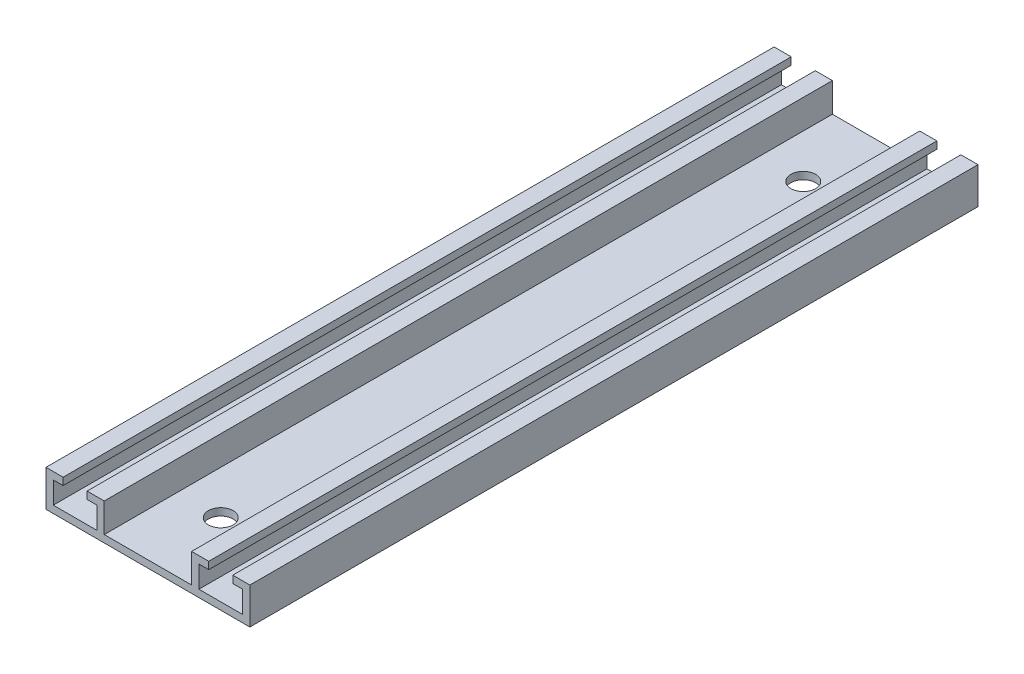
SolidWorks part; units mm, degrees
ref_plane "前视基准面" through (0, 0, 0) normal (0, 0, 1) x (1, 0, 0)
ref_plane "上视基准面" through (0, 0, 0) normal (0, 1, 0) x (1, 0, 0)
ref_plane "右视基准面" through (0, 0, 0) normal (1, 0, 0) x (0, 0, -1)
sketch "草图1" plane through (0, 0, 0) normal (0, 0, 1) x (1, 0, 0)
  line L0 (0, 0) -> (8, 0)
  line L1 (8, 0) -> (8, 5)
  line L2 (8, 5) -> (5.65, 5)
  line L3 (0, 0) -> (0, 5)
  line L4 (0, 5) -> (2.35, 5)
  line L5 (4, 0) -> (4, 6.7213) construction
  dimension "D1" = 3.3
  dimension "D2" = 8
  dimension "D3" = 5
extrude "拉伸-薄壁1" add sketch "草图1" along normal blind 100 thin thin type one direction wall 1
sketch "草图2" plane through (0, 0, 100) normal (0, 0, 1) x (1, 0, 0)
  line L0 (0, 0) -> (-6, 0)
  line L1 (8, 5) -> (8, 0) construction
  dimension "D1" = 14
extrude "拉伸-薄壁2" add sketch "草图2" against normal up to surface (100 mm away) thin
mirror "镜向1" about plane through (-6, 0, -6.0828) normal (1, 0, 0) of bodies 108
sketch "草图5" plane through (0, 1, 0) normal (0, 1, 0) x (1, 0, 0)
  line L0 (8, -50) -> (-25.3748, -50) construction
  line L1 (8, -100) -> (8, 0) construction
  line L3 (0, 0) -> (-12, 0) construction
  point P0 (-6, -90)
  point P2 (-6, -10)
  point P12 (-6, 0)
  dimension "D1" = 80
hole_wizard "M3 间隙孔1" positions "草图5" profile "草图4" hole size "M3" standard "GB" end condition through all
sketch "草图4" plane through (-6, 1, 90) normal (1, 0, 0) x (0, 0, 1)
  line L0 (0, 0) -> (0, 1)
  line L1 (0, 1) -> (1.7, 1)
  line L2 (1.7, 1) -> (1.7, 0)
  line L5 (1.7, 0) -> (0, 0)
  line L11 (0, -6.35) -> (0, 107.95) construction
  dimension "通孔孔直径" = 3.4
  dimension "通孔孔深度" = 1
